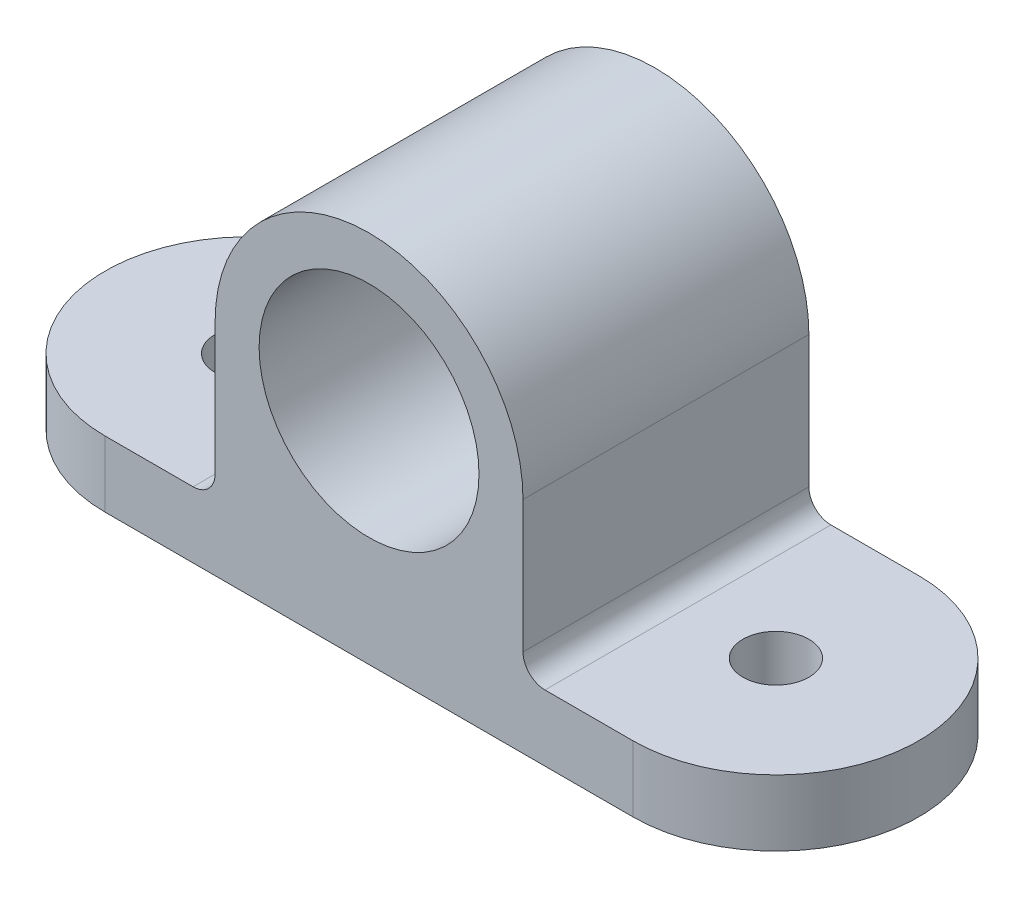
SolidWorks part; units mm, degrees
ref_plane "Front Plane" through (0, 0, 0) normal (0, 0, 1) x (1, 0, 0)
ref_plane "Top Plane" through (0, 0, 0) normal (0, 1, 0) x (1, 0, 0)
ref_plane "Right Plane" through (0, 0, 0) normal (1, 0, 0) x (0, 0, -1)
sketch "Sketch1" plane through (0, 0, 0) normal (0, 1, 0) x (1, 0, 0)
  line L0 (-24, 0) -> (24, 0) construction
  line L1 (-24, 13) -> (24, 13)
  line L2 (-24, -13) -> (24, -13)
  arc A0 (-24, 13) -> (-24, -13) centre (-24, 0) ccw
  arc A1 (24, -13) -> (24, 13) centre (24, 0) ccw
  circle A2 centre (-24, 0) radius 3
  circle A3 centre (24, 0) radius 3
  point P2 (0, 0)
  dimension "D2" = 13
  dimension "D3" = 6
  dimension "D4" = 6
  dimension "D1" = 48
extrude "Boss-Extrude1" add sketch "Sketch1" along normal blind 6
sketch "Sketch2" plane through (0, 0, 0) normal (0, 0, 1) x (1, 0, 0)
  line L0 (-14, 20) -> (-14, 0)
  line L1 (-24, 0) -> (24, 0) construction
  line L2 (-14, 0) -> (14, 0)
  line L3 (14, 20) -> (14, 0)
  circle A0 centre (0, 20) radius 10
  arc A1 (14, 20) -> (-14, 20) centre (0, 20) ccw
  dimension "D2" = 28
  dimension "D3" = 20
  dimension "D1" = 20
extrude "Boss-Extrude2" add sketch "Sketch2" along normal mid plane 26
fillet "Fillet1" radius 2 2 edges at (14, 6, 0) (-14, 6, 0)
